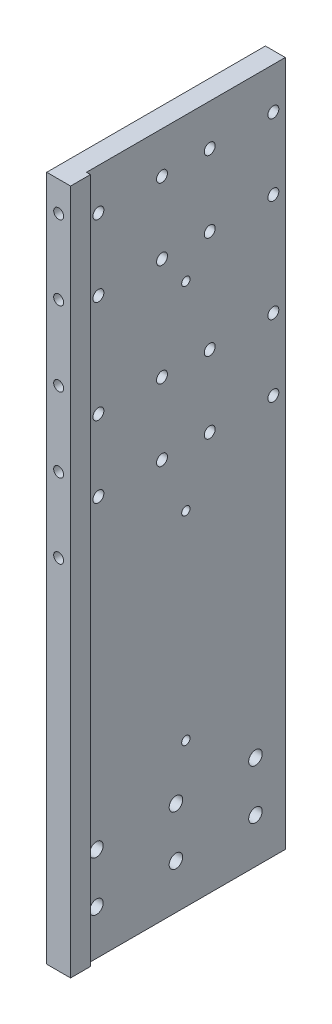
SolidWorks part; units mm, degrees
material "Q235A"
ref_plane "前视基准面" through (0, 0, 0) normal (0, 0, 1) x (1, 0, 0)
ref_plane "上视基准面" through (0, 0, 0) normal (0, 1, 0) x (1, 0, 0)
ref_plane "右视基准面" through (0, 0, 0) normal (1, 0, 0) x (0, 0, -1)
sketch "草图1" plane through (0, 0, 0) normal (1, 0, 0) x (0, 0, -1)
  line L1 (-55, -172.5) -> (55, -172.5)
  line L2 (-55, -172.5) -> (-55, 172.5)
  line L3 (-55, 172.5) -> (55, 172.5)
  line L4 (55, -172.5) -> (55, 172.5)
  line L5 (-55, -172.5) -> (55, 172.5) construction
  line L6 (-55, 172.5) -> (55, -172.5) construction
  point P0 (0, 0)
  dimension "D1" = 110
  dimension "D2" = 345
extrude "凸台-拉伸1" add sketch "草图1" along normal mid plane 12
sketch "草图2" plane through (6, 0, 0) normal (1, 0, 0) x (0, 0, -1)
  line L0 (-55, -172.5) -> (55, -172.5) construction
  line L1 (-45, 172.5) -> (55, 172.5)
  line L2 (-45, 172.5) -> (-45, -172.5)
  line L3 (-45, -172.5) -> (55, -172.5)
  line L4 (55, 172.5) -> (55, -172.5)
  line L5 (-55, 172.5) -> (-55, -172.5) construction
  dimension "D1" = 10
extrude "切除-拉伸1" cut sketch "草图2" against normal blind 2
hole_wizard "M5 六角凹头螺钉的柱形沉头孔1" positions "草图3" profile "草图4" counterbore size "M5" standard "ISO" end condition through all
sketch "草图3" plane through (-6, 0, 0) normal (-1, 0, 0) x (0, 0, 1)
  line L1 (-55, -172.5) -> (-55, 172.5) construction
  line L2 (-55, 172.5) -> (55, 172.5) construction
  point P0 (-49, 151.75)
  point P3 (-17, 151.75)
  point P6 (7, 151.75)
  point P9 (39, 151.75)
  point P12 (39, 115.75)
  point P15 (7, 115.75)
  point P18 (-17, 115.75)
  point P21 (-49, 115.75)
  point P24 (-49, 64.25)
  point P27 (-49, 28.25)
  point P30 (-17, 64.25)
  point P33 (-17, 28.25)
  point P36 (7, 64.25)
  point P39 (-17, 28.25)
  point P41 (7, 28.25)
  point P44 (39, 64.25)
  point P47 (39, 28.25)
  dimension "D1" = 32
  dimension "D2" = 56
  dimension "D3" = 88
  dimension "D4" = 36
  dimension "D5" = 87.5
  dimension "D6" = 123.5
  dimension "D7" = 6
  dimension "D8" = 20.75
sketch "草图4" plane through (-6, 151.75, -49) normal (0, 1, 0) x (0, 0, 1)
  line L0 (0, 0) -> (0, 12)
  line L1 (0, 12) -> (2.75, 12)
  line L3 (2.75, 12) -> (2.75, 5.4)
  line L4 (2.75, 5.4) -> (5, 5.4)
  line L5 (5, 5.4) -> (5, 0)
  line L7 (5, 0) -> (0, 0)
  line L11 (0, -6.35) -> (0, 107.95) construction
  dimension "通孔孔直径" = 5.5
  dimension "通孔孔深度" = 12
  dimension "柱形沉头孔直径" = 10
  dimension "柱形沉头孔深度" = 5.4
hole_wizard "M8 螺纹孔1" positions "草图5" profile "草图6" tap size "M8" standard "ISO" end condition through all
sketch "草图5" plane through (-6, 0, 0) normal (-1, 0, 0) x (0, 0, 1)
  line L0 (55, -172.5) -> (-55, -172.5) construction
  point P0 (-40, -125)
  point P3 (-40, -150)
  point P6 (0, -125)
  point P9 (0, -150)
  point P12 (40, -125)
  point P15 (40, -150)
  dimension "D1" = 40
  dimension "D2" = 40
  dimension "D3" = 25
  dimension "D4" = 47.5
sketch "草图6" plane through (-6, -125, -40) normal (0, 1, 0) x (0, 0, 1)
  line L0 (0, 0) -> (0, 12)
  line L1 (0, 12) -> (3.4, 12)
  line L2 (3.4, 12) -> (3.4, 0)
  line L5 (3.4, 0) -> (0, 0)
  line L11 (0, -6.35) -> (0, 107.95) construction
  dimension "通孔螺纹孔钻头直径" = 6.8
  dimension "通孔螺纹孔钻头深度" = 12
cosmetic thread "孔螺蚊线1" parameters "D2"=8
cosmetic thread "孔螺蚊线2" parameters "D2"=8
cosmetic thread "孔螺蚊线3" parameters "D2"=8
cosmetic thread "孔螺蚊线4" parameters "D2"=8
cosmetic thread "孔螺蚊线5" parameters "D2"=8
cosmetic thread "孔螺蚊线6" parameters "D2"=8
hole_wizard "M6 螺纹孔1" positions "草图9" profile "草图8" tap size "M6" standard "ISO"
sketch "草图9" plane through (0, 0, 55) normal (0, 0, 1) x (1, 0, 0)
  line L3 (6, 172.5) -> (-6, 172.5) construction
  point P0 (0, 7.5)
  point P3 (0, 45)
  point P6 (0, 82.5)
  point P9 (0, 120)
  point P12 (0, 157.5)
  dimension "D1" = 37.5
  dimension "D2" = 75
  dimension "D3" = 112.5
  dimension "D4" = 150
  dimension "D5" = 15
sketch "草图8" plane through (0, 7.5, 55) normal (1, 0, 0) x (0, -1, 0)
  line L0 (0, 0) -> (0, 16.5022)
  line L1 (0, 16.5022) -> (2.5, 15)
  line L2 (2.5, 15) -> (2.5, 0)
  line L5 (2.5, 0) -> (0, 0)
  line L10 (0, 16.5022) -> (-2.5, 15) construction
  line L11 (0, -6.35) -> (0, 107.95) construction
  dimension "螺纹孔钻头直径" = 5
  dimension "螺纹孔钻头深度" = 15
  dimension "导头角度" = 118
cosmetic thread "孔螺蚊线8" parameters "D1"=12, "D2"=6
cosmetic thread "孔螺蚊线9" parameters "D1"=12, "D2"=6
cosmetic thread "孔螺蚊线10" parameters "D1"=12, "D2"=6
cosmetic thread "孔螺蚊线11" parameters "D1"=12, "D2"=6
cosmetic thread "孔螺蚊线17" parameters "D1"=12, "D2"=6
hole_wizard "M5 螺纹孔1" positions "草图10" profile "草图11" tap size "M5" standard "ISO" end condition through all
sketch "草图10" plane through (-6, 0, 0) normal (-1, 0, 0) x (0, 0, 1)
  line L0 (-55, -172.5) -> (-55, 172.5) construction
  point P0 (-5, 185)
  point P3 (-5, 100)
  point P6 (-5, 0)
  point P9 (-5, -100)
  dimension "D1" = 50
  dimension "D2" = 100
  dimension "D3" = 100
  dimension "D4" = 85
sketch "草图11" plane through (-6, 185, -5) normal (0, 1, 0) x (0, 0, 1)
  line L0 (0, 0) -> (0, 12)
  line L1 (0, 12) -> (2.1, 12)
  line L2 (2.1, 12) -> (2.1, 0)
  line L5 (2.1, 0) -> (0, 0)
  line L11 (0, -6.35) -> (0, 107.95) construction
  dimension "通孔螺纹孔钻头直径" = 4.2
  dimension "通孔螺纹孔钻头深度" = 12
cosmetic thread "孔螺蚊线13" parameters "D2"=5
cosmetic thread "孔螺蚊线14" parameters "D2"=5
cosmetic thread "孔螺蚊线15" parameters "D2"=5
